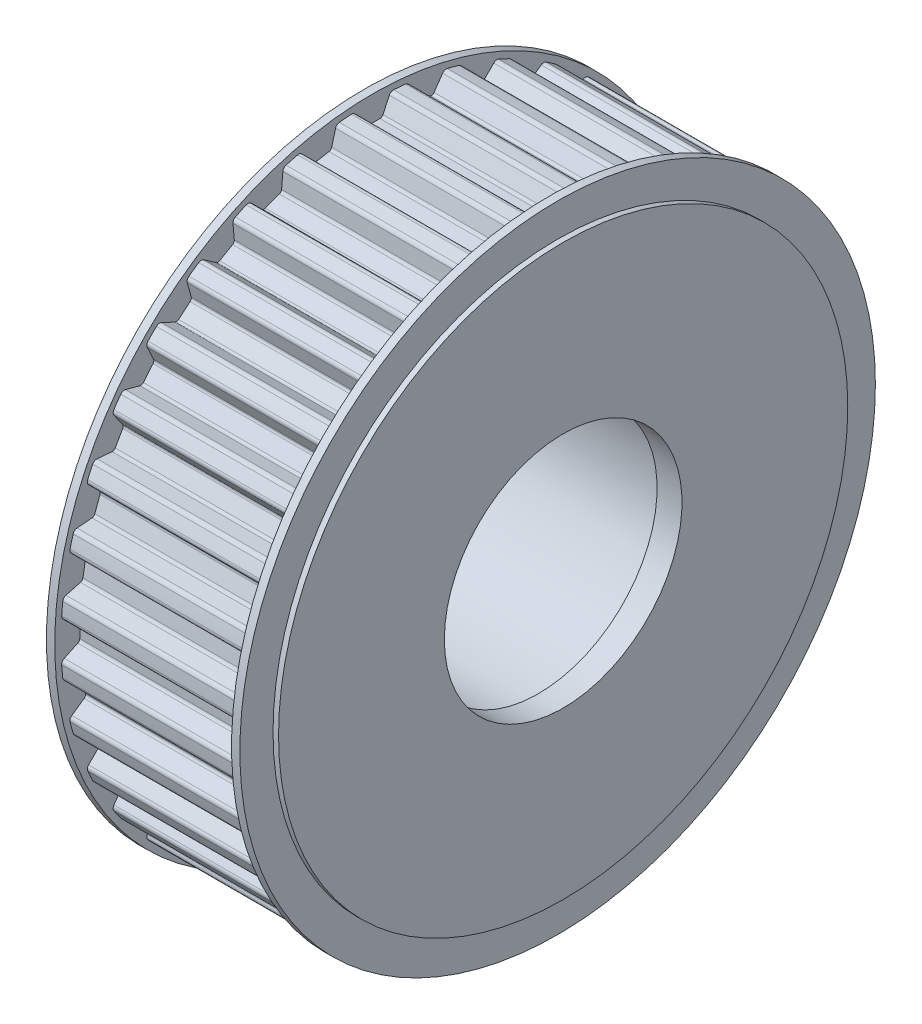
from build123d import *

# Parameters (mm, degrees)
SKETCH_1_R                       = 56.37
EXTRUDE_1_DEPTH                  = 16
CUT_EXTRUDE_2_DEPTH              = 32
FILLET_1_R                       = 0.6
FILLET_2_R                       = 0.8
PATTERN_CIRCULAR_1_COUNT         = 36
FILLET_1_OF_PATTERN_CIRCULAR_1_R = 0.6
FILLET_2_OF_PATTERN_CIRCULAR_1_R = 0.8
SKETCH_6_R                       = 57.5
EXTRUDE_2_DEPTH                  = 1.5
SKETCH_7_R                       = 51.5
EXTRUDE_3_DEPTH                  = 1
SKETCH_8_R                       = 21.5
CUT_EXTRUDE_1_DEPTH              = 90.339241098
SKETCH_9_R                       = 23.5
CUT_EXTRUDE_2_2_DEPTH            = 32.5
SKETCH_10_W                      = 1.8
SKETCH_10_H                      = 1.25


with BuildPart() as part:
    # 草图1 → 拉伸1 (new, symmetric)
    with BuildSketch(Plane(origin=(0, 0, 0), x_dir=(0, 0, -1), z_dir=(1, 0, 0))):
        Circle(SKETCH_1_R)
    extrude(amount=EXTRUDE_1_DEPTH, both=True)

    # 草图2 → Cut-Extrude 2 (cut)
    with BuildSketch(Plane(origin=(16, 0, 0), x_dir=(0, 0, -1), z_dir=(1, 0, 0))):
        with BuildLine():
            Line((-3.285, 56.274200794), (-1.744225866, 52.97))
            Line((-1.744225866, 52.97), (1.744225866, 52.97))
            Line((1.744225866, 52.97), (3.285, 56.274200794))
            ThreePointArc((3.285, 56.274200794), (0, 56.37), (-3.285, 56.274200794))
        make_face()
    cut_extrude_2 = extrude(amount=-CUT_EXTRUDE_2_DEPTH, mode=Mode.SUBTRACT)

    # 圆角1
    fillet_1_edges = [part.edges().sort_by_distance(p)[0] for p in [
        (0, 52.97, 1.744225866),
        (0, 52.97, -1.744225866),
    ]]
    fillet(fillet_1_edges, radius=FILLET_1_R)

    # 圆角2
    fillet_2_edges = [part.edges().sort_by_distance(p)[0] for p in [
        (0, 56.274200794, 3.285),
        (0, 56.274200794, -3.285),
    ]]
    fillet(fillet_2_edges, radius=FILLET_2_R)

    # 阵列(圆周)1: Cut-Extrude 2 ×36 about axis
    pattern_circular_1_axis = Axis((0, 0, 0), (1, 0, 0))
    for i in range(1, PATTERN_CIRCULAR_1_COUNT):
        add(cut_extrude_2.rotate(pattern_circular_1_axis, i * 360 / PATTERN_CIRCULAR_1_COUNT), mode=Mode.SUBTRACT)

    # 圆角1 of 阵列(圆周)1
    fillet_1_of_pattern_circular_1_edges = [part.edges().sort_by_distance(p)[0] for p in [
        (0, 51.862385034, 10.915871127),
        (0, 52.46814832, 7.480416815),
        (0, 49.178957742, 19.755843167),
        (0, 50.372078504, 16.477770817),
        (0, 45.001252706, 27.99554391),
        (0, 46.745478571, 24.97445609),
        (0, 39.456207377, 35.384614217),
        (0, 41.698540927, 32.712305153),
        (0, 32.712305153, 41.698540927),
        (0, 35.384614217, 39.456207377),
        (0, 24.97445609, 46.745478571),
        (0, 27.99554391, 45.001252706),
        (0, 16.477770817, 50.372078504),
        (0, 19.755843167, 49.178957742),
        (0, 7.480416815, 52.46814832),
        (0, 10.915871127, 51.862385034),
        (0, -1.744225866, 52.97),
        (0, 1.744225866, 52.97),
        (0, -10.915871127, 51.862385034),
        (0, -7.480416815, 52.46814832),
        (0, -19.755843167, 49.178957742),
        (0, -16.477770817, 50.372078504),
        (0, -27.99554391, 45.001252706),
        (0, -24.97445609, 46.745478571),
        (0, -35.384614217, 39.456207377),
        (0, -32.712305153, 41.698540927),
        (0, -41.698540927, 32.712305153),
        (0, -39.456207377, 35.384614217),
        (0, -46.745478571, 24.97445609),
        (0, -45.001252706, 27.99554391),
        (0, -50.372078504, 16.477770817),
        (0, -49.178957742, 19.755843167),
        (0, -52.46814832, 7.480416815),
        (0, -51.862385034, 10.915871127),
        (0, -52.97, -1.744225866),
        (0, -52.97, 1.744225866),
        (0, -51.862385034, -10.915871127),
        (0, -52.46814832, -7.480416815),
        (0, -49.178957742, -19.755843167),
        (0, -50.372078504, -16.477770817),
        (0, -45.001252706, -27.99554391),
        (0, -46.745478571, -24.97445609),
        (0, -39.456207377, -35.384614217),
        (0, -41.698540927, -32.712305153),
        (0, -32.712305153, -41.698540927),
        (0, -35.384614217, -39.456207377),
        (0, -24.97445609, -46.745478571),
        (0, -27.99554391, -45.001252706),
        (0, -16.477770817, -50.372078504),
        (0, -19.755843167, -49.178957742),
        (0, -7.480416815, -52.46814832),
        (0, -10.915871127, -51.862385034),
        (0, 1.744225866, -52.97),
        (0, -1.744225866, -52.97),
        (0, 10.915871127, -51.862385034),
        (0, 7.480416815, -52.46814832),
        (0, 19.755843167, -49.178957742),
        (0, 16.477770817, -50.372078504),
        (0, 27.99554391, -45.001252706),
        (0, 24.97445609, -46.745478571),
        (0, 35.384614217, -39.456207377),
        (0, 32.712305153, -41.698540927),
        (0, 41.698540927, -32.712305153),
        (0, 39.456207377, -35.384614217),
        (0, 46.745478571, -24.97445609),
        (0, 45.001252706, -27.99554391),
        (0, 50.372078504, -16.477770817),
        (0, 49.178957742, -19.755843167),
        (0, 52.46814832, -7.480416815),
        (0, 51.862385034, -10.915871127),
    ]]
    fillet(fillet_1_of_pattern_circular_1_edges, radius=FILLET_1_OF_PATTERN_CIRCULAR_1_R)

    # 圆角2 of 阵列(圆周)1
    fillet_2_of_pattern_circular_1_edges = [part.edges().sort_by_distance(p)[0] for p in [
        (0, 54.848834973, 13.007005886),
        (0, 55.9897035, 6.536818949),
        (0, 51.756915056, 22.33380048),
        (0, 54.003987398, 16.160019962),
        (0, 47.092387465, 30.981993848),
        (0, 50.377387465, 25.292206946),
        (0, 40.996981511, 38.688815011),
        (0, 45.220096107, 33.65590302),
        (0, 33.65590302, 45.220096107),
        (0, 38.688815011, 40.996981511),
        (0, 25.292206946, 50.377387465),
        (0, 30.981993848, 47.092387465),
        (0, 16.160019962, 54.003987398),
        (0, 22.33380048, 51.756915056),
        (0, 6.536818949, 55.9897035),
        (0, 13.007005886, 54.848834973),
        (0, -3.285, 56.274200794),
        (0, 3.285, 56.274200794),
        (0, -13.007005886, 54.848834973),
        (0, -6.536818949, 55.9897035),
        (0, -22.33380048, 51.756915056),
        (0, -16.160019962, 54.003987398),
        (0, -30.981993848, 47.092387465),
        (0, -25.292206946, 50.377387465),
        (0, -38.688815011, 40.996981511),
        (0, -33.65590302, 45.220096107),
        (0, -45.220096107, 33.65590302),
        (0, -40.996981511, 38.688815011),
        (0, -50.377387465, 25.292206946),
        (0, -47.092387465, 30.981993848),
        (0, -54.003987398, 16.160019962),
        (0, -51.756915056, 22.33380048),
        (0, -55.9897035, 6.536818949),
        (0, -54.848834973, 13.007005886),
        (0, -56.274200794, -3.285),
        (0, -56.274200794, 3.285),
        (0, -54.848834973, -13.007005886),
        (0, -55.9897035, -6.536818949),
        (0, -51.756915056, -22.33380048),
        (0, -54.003987398, -16.160019962),
        (0, -47.092387465, -30.981993848),
        (0, -50.377387465, -25.292206946),
        (0, -40.996981511, -38.688815011),
        (0, -45.220096107, -33.65590302),
        (0, -33.65590302, -45.220096107),
        (0, -38.688815011, -40.996981511),
        (0, -25.292206946, -50.377387465),
        (0, -30.981993848, -47.092387465),
        (0, -16.160019962, -54.003987398),
        (0, -22.33380048, -51.756915056),
        (0, -6.536818949, -55.9897035),
        (0, -13.007005886, -54.848834973),
        (0, 3.285, -56.274200794),
        (0, -3.285, -56.274200794),
        (0, 13.007005886, -54.848834973),
        (0, 6.536818949, -55.9897035),
        (0, 22.33380048, -51.756915056),
        (0, 16.160019962, -54.003987398),
        (0, 30.981993848, -47.092387465),
        (0, 25.292206946, -50.377387465),
        (0, 38.688815011, -40.996981511),
        (0, 33.65590302, -45.220096107),
        (0, 45.220096107, -33.65590302),
        (0, 40.996981511, -38.688815011),
        (0, 50.377387465, -25.292206946),
        (0, 47.092387465, -30.981993848),
        (0, 54.003987398, -16.160019962),
        (0, 51.756915056, -22.33380048),
        (0, 55.9897035, -6.536818949),
        (0, 54.848834973, -13.007005886),
    ]]
    fillet(fillet_2_of_pattern_circular_1_edges, radius=FILLET_2_OF_PATTERN_CIRCULAR_1_R)

    # 草图6 → 凸台-拉伸2 (add)
    with BuildSketch(Plane(origin=(16, 0, 0), x_dir=(0, 0, -1), z_dir=(1, 0, 0))):
        Circle(SKETCH_6_R)
    extrude_2 = extrude(amount=EXTRUDE_2_DEPTH)

    # 草图7 → 凸台-拉伸3 (add)
    with BuildSketch(Plane(origin=(17.5, 0, 0), x_dir=(0, 0, -1), z_dir=(1, 0, 0))):
        Circle(SKETCH_7_R)
    extrude_3 = extrude(amount=EXTRUDE_3_DEPTH)

    # 镜向2: 凸台-拉伸2, 凸台-拉伸3 across plane
    add(extrude_2.mirror(Plane(origin=(0, 0, 0), x_dir=(0, 0, 1), z_dir=(1, 0, 0))))
    add(extrude_3.mirror(Plane(origin=(0, 0, 0), x_dir=(0, 0, 1), z_dir=(1, 0, 0))))

    # 草图8 → 切除-拉伸1 (cut, through all)
    with BuildSketch(Plane.ZY.offset(18.5)):
        Circle(SKETCH_8_R)
    extrude(amount=-CUT_EXTRUDE_1_DEPTH, mode=Mode.SUBTRACT)

    # 草图9 → Cut-Extrude 2 2 (cut)
    with BuildSketch(Plane.ZY.offset(18.5)):
        Circle(SKETCH_9_R)
    extrude(amount=-CUT_EXTRUDE_2_2_DEPTH, mode=Mode.SUBTRACT)

    # 草图10 → 切除-旋转1 (revolve, cut)
    with BuildSketch(Plane(origin=(0, 0, 0), x_dir=(1, 0, 0), z_dir=(0, 1, 0)), mode=Mode.PRIVATE) as cut_revolve_1_sk:
        with Locations((-14.9, 24.125)):
            Rectangle(SKETCH_10_W, SKETCH_10_H)
    revolve(cut_revolve_1_sk.sketch.rotate(Axis((0, 0, 0), (-1, 0, 0)), 180), axis=Axis((0, 0, 0), (-1, 0, 0)), mode=Mode.SUBTRACT)


solid = part.part
